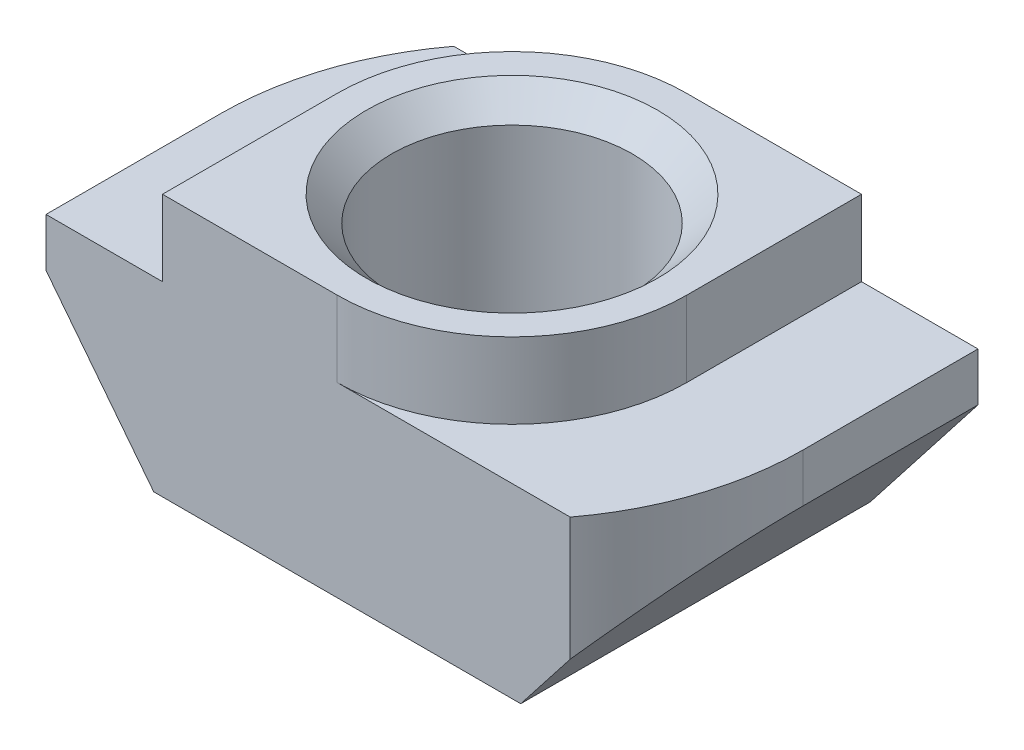
from build123d import *

# Parameters (mm, degrees)
EXTRUDE_1_DEPTH     = 6
CUT_EXTRUDE_1_DEPTH = 4.5
CUT_EXTRUDE_2_DEPTH = 4.5
FILLET_1_R          = 3


with BuildPart() as part:
    # 草图1 → 凸台-拉伸1 (new body)
    with BuildSketch(Plane.XY):
        Polygon((-5, 2.36789202), (-3.15, 0), (3.15, 0), (5, 2.36789202), (5, 3.2), (3, 3.2), (3, 4.5), (-3, 4.5), (-3, 3.2), (-5, 3.2), align=None)
    extrude(amount=EXTRUDE_1_DEPTH)

    # 草图2 → 切除-旋转1 (revolve, cut)
    with BuildSketch(Plane(origin=(0, 0, 0), x_dir=(0, 0, -1), z_dir=(1, 0, 0)), mode=Mode.PRIVATE) as cut_revolve_1_sk:
        Polygon((-3, 0), (-5.5, 0), (-5.067, 0.433), (-5.067, 4.067), (-5.5, 4.5), (-3, 4.5), align=None)
    revolve(cut_revolve_1_sk.sketch.rotate(Axis((0, 50, 3), (0, -1, 0)), 180), axis=Axis((0, 50, 3), (0, -1, 0)), mode=Mode.SUBTRACT)

    # 草图3 → 切除-拉伸1 (cut)
    with BuildSketch(Plane(origin=(0, 4.5, 0), x_dir=(1, 0, 0), z_dir=(0, 1, 0))):
        with BuildLine():
            Line((4, -6), (5, -6))
            Line((5, -6), (5, -3))
            ThreePointArc((5, -3), (4.74341649, -4.58113883), (4, -6))
        make_face()
    extrude(amount=-CUT_EXTRUDE_1_DEPTH, mode=Mode.SUBTRACT)

    # 草图4 → 切除-拉伸2 (cut)
    with BuildSketch(Plane(origin=(0, 4.5, 0), x_dir=(1, 0, 0), z_dir=(0, 1, 0))):
        with BuildLine():
            Line((-4, 0), (-5, 0))
            Line((-5, 0), (-5, -3))
            ThreePointArc((-5, -3), (-4.74341649, -1.41886117), (-4, 0))
        make_face()
    extrude(amount=-CUT_EXTRUDE_2_DEPTH, mode=Mode.SUBTRACT)

    # 圆角1
    fillet_1_edges = [part.edges().sort_by_distance(p)[0] for p in [
        (3, 3.85, 6),
        (-3, 3.85, 0),
    ]]
    fillet(fillet_1_edges, radius=FILLET_1_R)


solid = part.part
